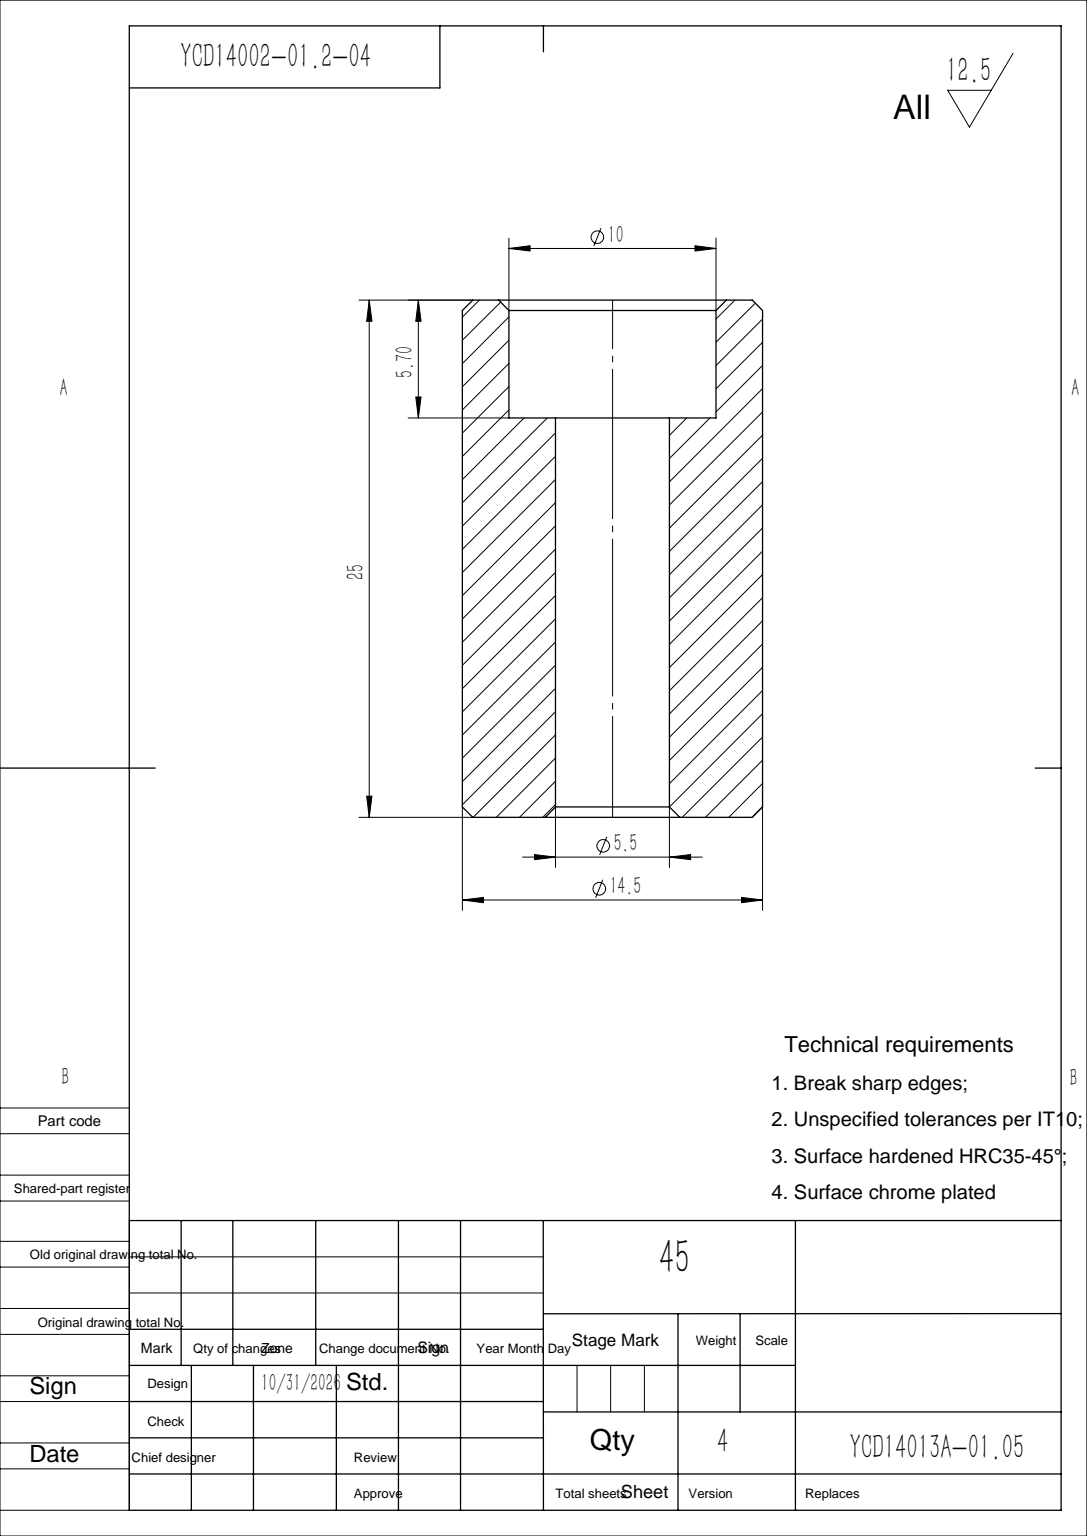
from build123d import *

# Parameters (mm, degrees)
SKETCH1_R                                       = 7.25
BOSS_EXTRUDE1_DEPTH                             = 25
HOLE_SIZE_BY_HEX_SOCKET_SCREW_TYPE1_D           = 5.5
HOLE_SIZE_BY_HEX_SOCKET_SCREW_TYPE1_CBORE_D     = 10
HOLE_SIZE_BY_HEX_SOCKET_SCREW_TYPE1_CBORE_DEPTH = 5.7
CHAMFER1_SIZE                                   = 0.5


with BuildPart() as part:
    # Sketch1 → Boss-Extrude1 (new body)
    with BuildSketch(Plane(origin=(0, 0, 0), x_dir=(1, 0, 0), z_dir=(0, 1, 0))):
        with Locations(Location((0, 0, 0), (0, 0, 270))):
            Circle(SKETCH1_R)
    extrude(amount=BOSS_EXTRUDE1_DEPTH)

    # Hole Size by Hex Socket Screw Type1 (through all)
    with Locations(Plane(origin=(0, 25, 0), x_dir=(1, 0, 0), z_dir=(0, 1, 0))):
        with Locations((0, 0)):
            CounterBoreHole(HOLE_SIZE_BY_HEX_SOCKET_SCREW_TYPE1_D / 2, HOLE_SIZE_BY_HEX_SOCKET_SCREW_TYPE1_CBORE_D / 2, HOLE_SIZE_BY_HEX_SOCKET_SCREW_TYPE1_CBORE_DEPTH)

    # Chamfer1
    chamfer1_edges = [part.edges().sort_by_distance(p)[0] for p in [
        (0, 0, -7.25),
        (0, 25, -7.25),
        (-5, 25, 0),
        (2.75, 0, 0),
    ]]
    chamfer(chamfer1_edges, length=CHAMFER1_SIZE)


solid = part.part
